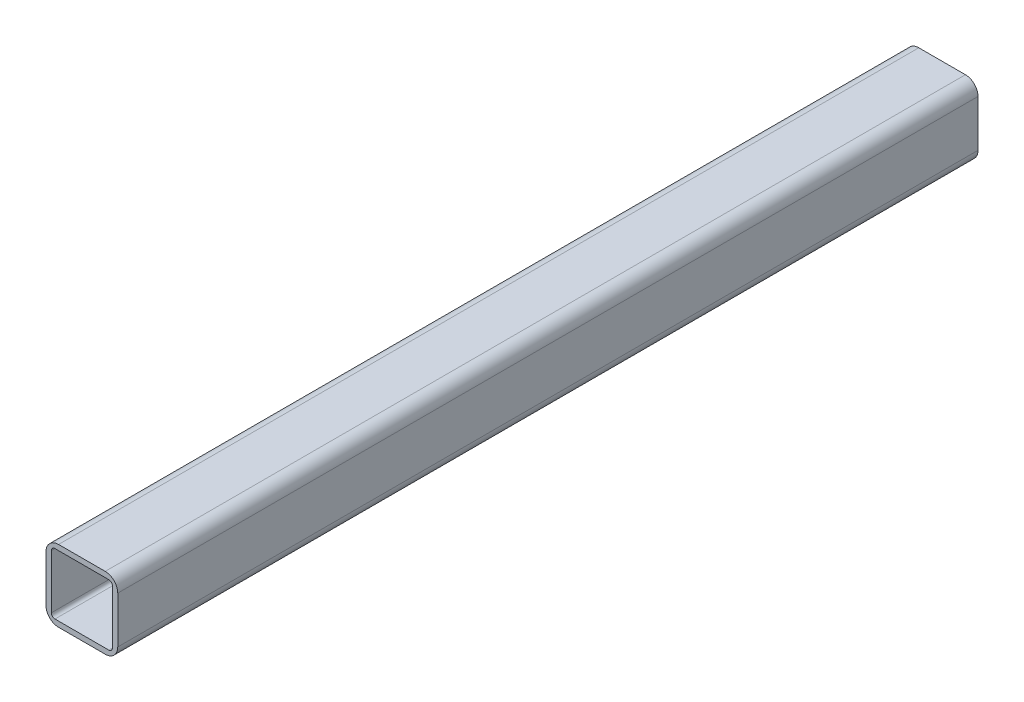
from build123d import *

# Parameters (mm, degrees)
SKETCH1_W           = 40
SKETCH1_H           = 40
SKETCH1_W_2         = 34
SKETCH1_H_2         = 34
BOSS_EXTRUDE1_DEPTH = 479.48
FILLET1_R           = 2
FILLET2_R           = 7


with BuildPart() as part:
    # Sketch1 → Boss-Extrude1 (new body)
    with BuildSketch(Plane.XY):
        Rectangle(SKETCH1_W, SKETCH1_H)
        Rectangle(SKETCH1_W_2, SKETCH1_H_2, mode=Mode.SUBTRACT)
    extrude(amount=BOSS_EXTRUDE1_DEPTH)

    # Fillet1
    fillet1_edges = [part.edges().sort_by_distance(p)[0] for p in [
        (17, -17, 239.74),
        (17, 17, 239.74),
        (-17, 17, 239.74),
        (-17, -17, 239.74),
    ]]
    fillet(fillet1_edges, radius=FILLET1_R)

    # Fillet2
    fillet2_edges = [part.edges().sort_by_distance(p)[0] for p in [
        (20, -20, 239.74),
        (-20, -20, 239.74),
        (-20, 20, 239.74),
        (20, 20, 239.74),
    ]]
    fillet(fillet2_edges, radius=FILLET2_R)


solid = part.part
